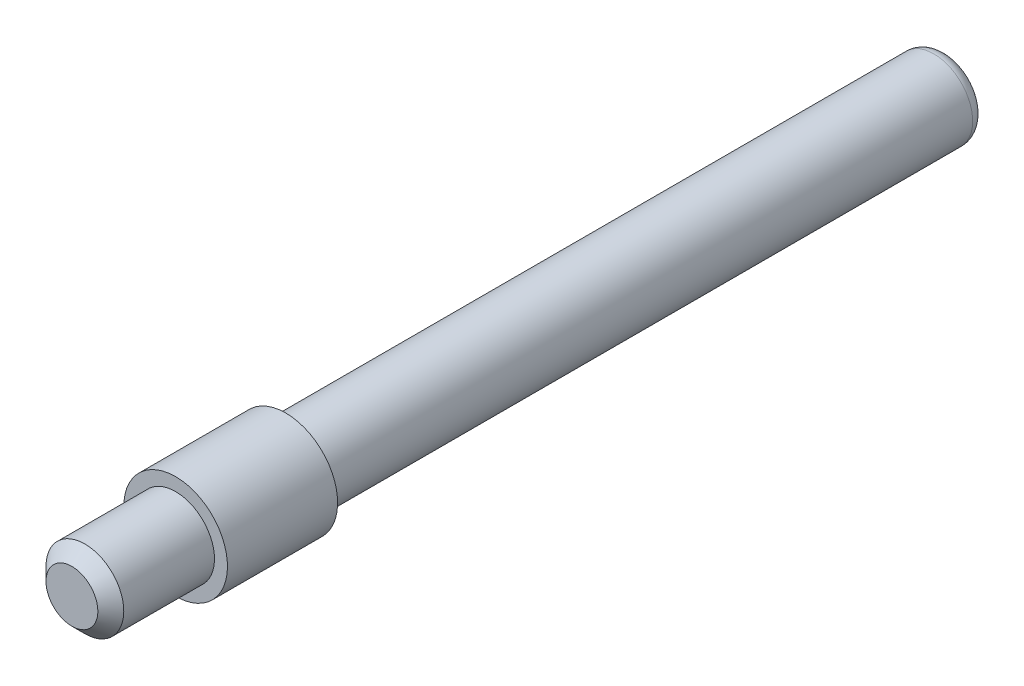
from build123d import *

# Parameters (mm, degrees)
FILLET_1_R     = 1
CHAMFER_1_SIZE = 1


with BuildPart() as part:
    # 草图1 → 旋转1 (revolve)
    with BuildSketch(Plane(origin=(0, 0, 0), x_dir=(0, 0, -1), z_dir=(1, 0, 0))):
        Polygon((0, 0), (0, 3), (8, 3), (8, 4), (16.5, 4), (16.5, 3), (67.5, 3), (67.5, 0), align=None)
    revolve(axis=Axis((0, 0, -67.5), (0, 0, 1)))

    # 圆角1
    fillet_1_edges = [part.edges().sort_by_distance(p)[0] for p in [
        (0, -3, -67.5),
    ]]
    fillet(fillet_1_edges, radius=FILLET_1_R)

    # 倒角1
    chamfer_1_edges = [part.edges().sort_by_distance(p)[0] for p in [
        (0, -3, 0),
    ]]
    chamfer(chamfer_1_edges, length=CHAMFER_1_SIZE)


solid = part.part
